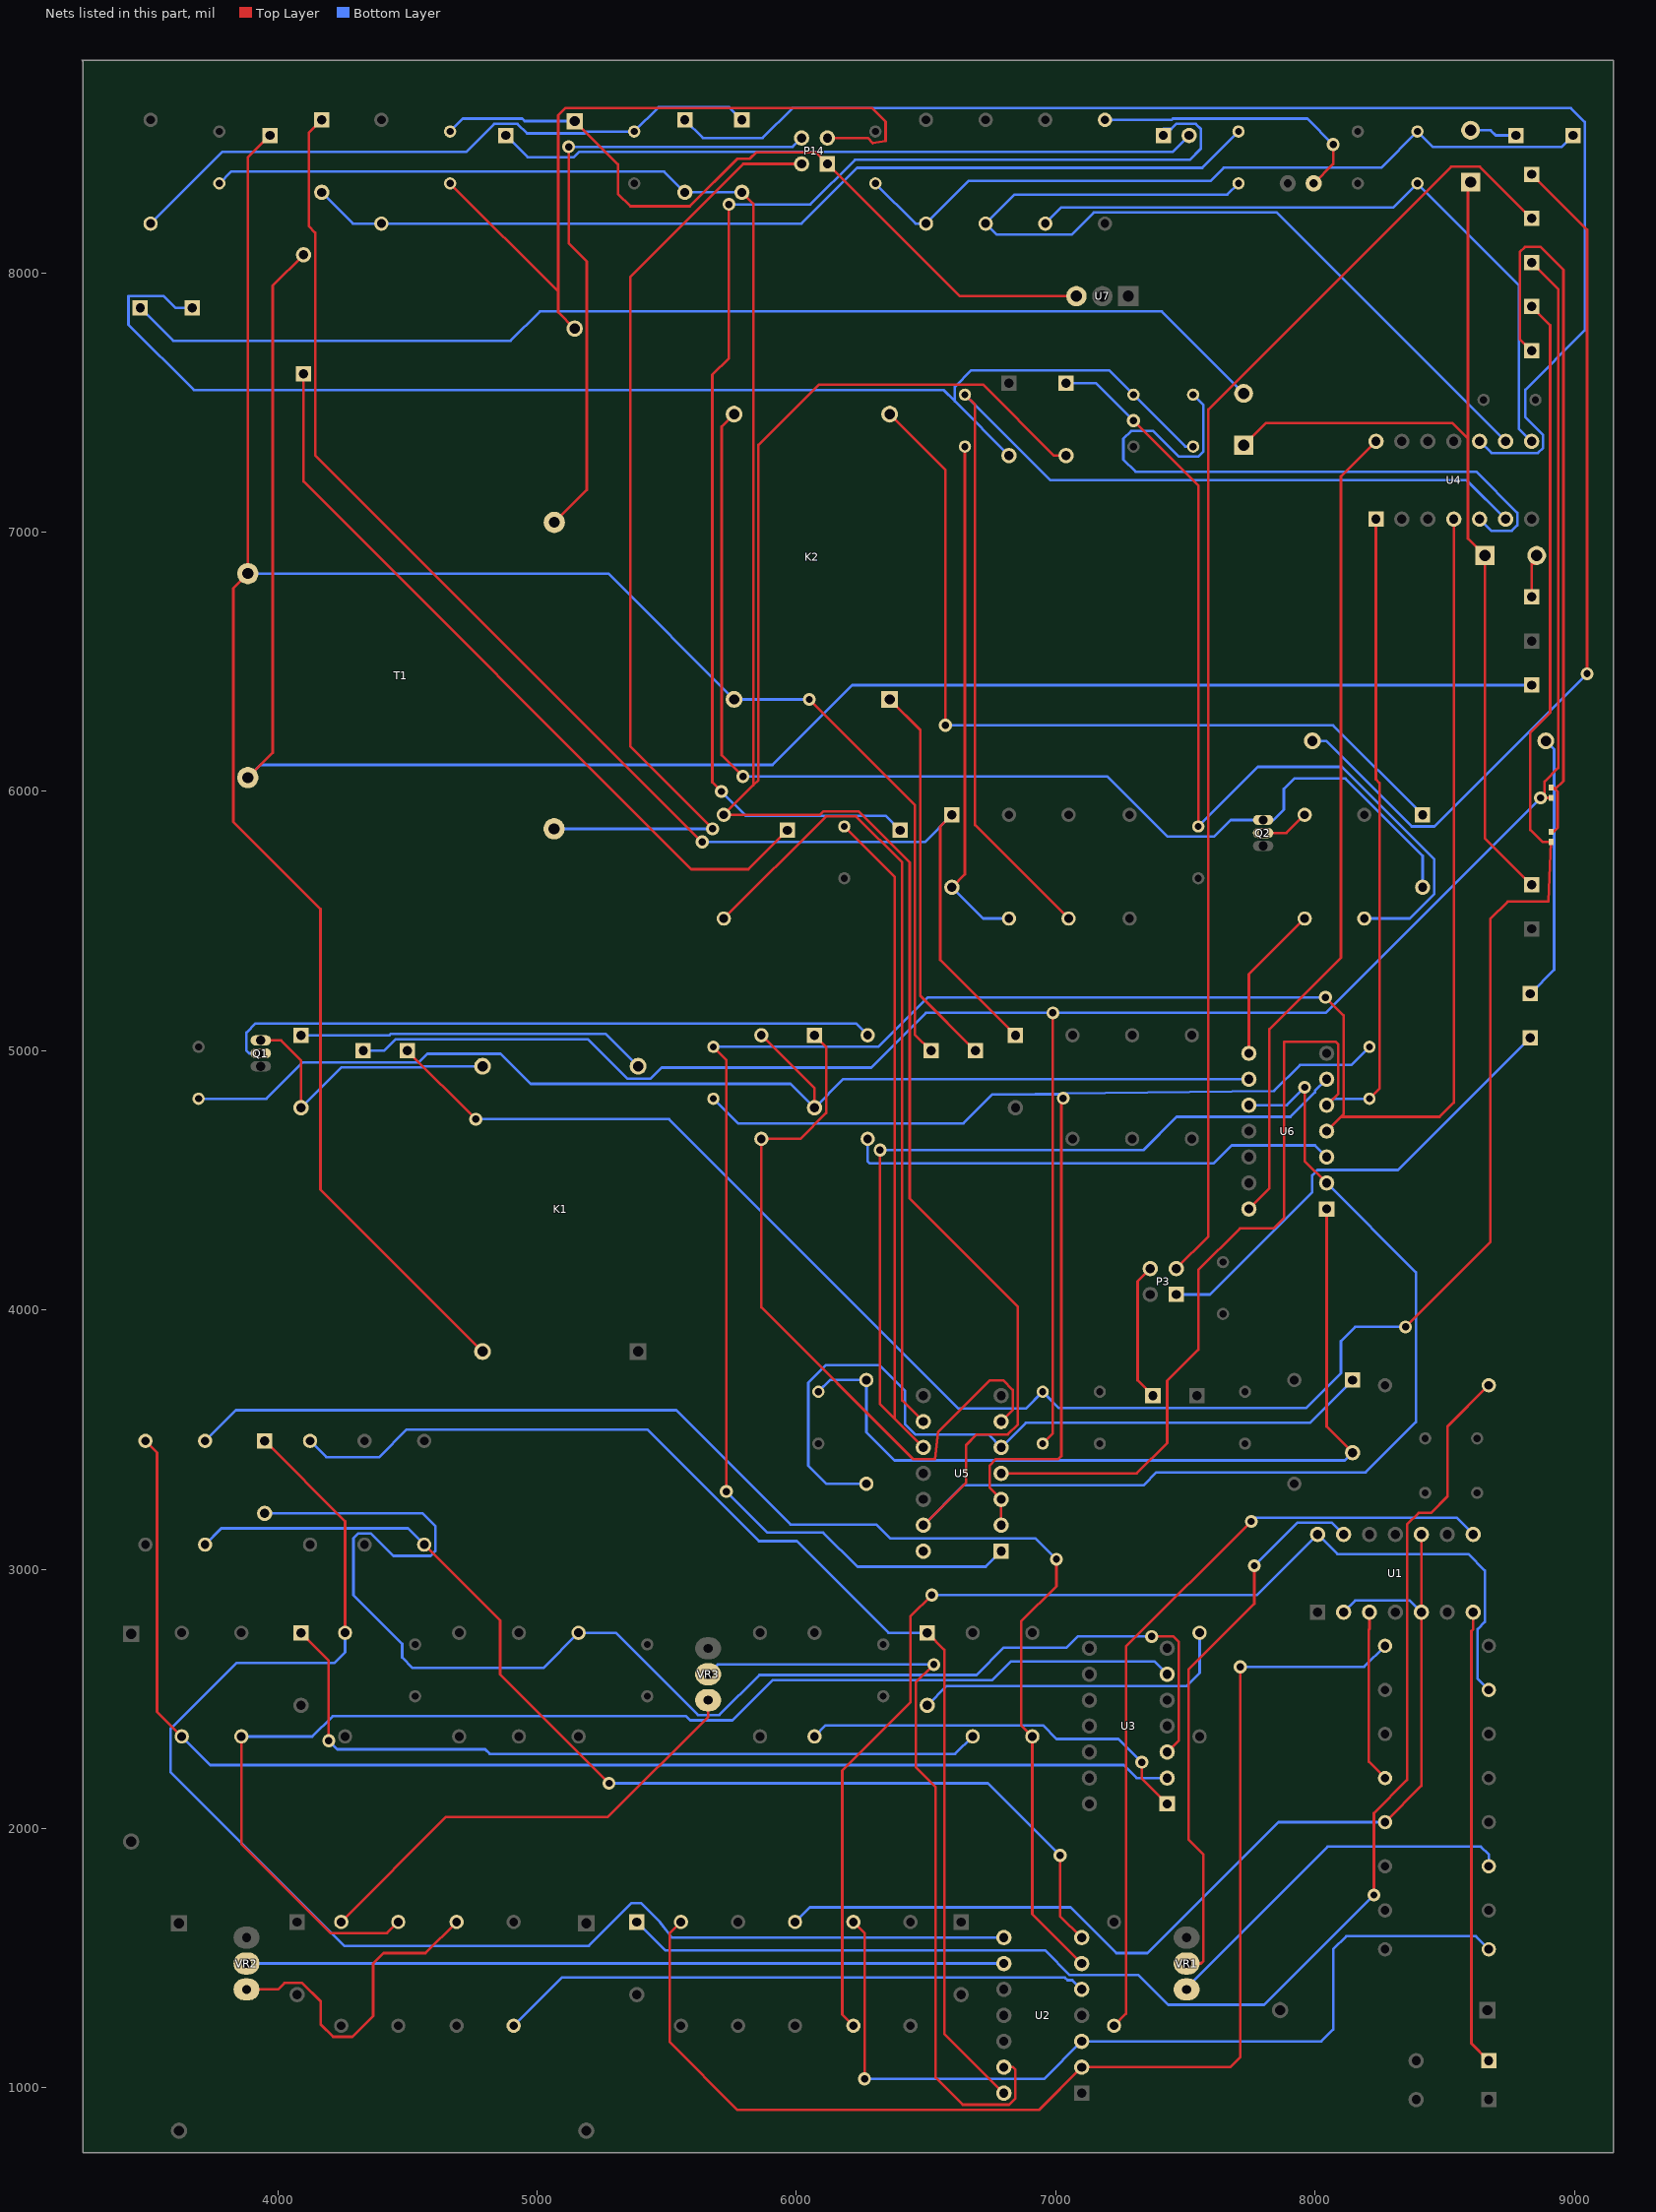
[diagram p0: the nets of this part, all layers, seen from the top]
# Altium PCB MISC82089.PcbDoc (part 2 of 2)
Units mil, origin at the board's own origin, x right, y up, seen from the top; angles counter-clockwise.
Board outline 5905 x 8070 mil, 2 copper layers (Top Layer, Bottom Layer); 156 components, 100 nets, 374 pads, 37 vias.

## Via types
v1: diameter 50, hole 28, Top Layer to Bottom Layer, 37 vias

## Nets (pads, with @x,y where several pads share a name; then routed paths per layer and width w, separated by ;. In a path a pad name is that pad's centre, name@x,y a point inside that pad or via, vN(x,y) a via of type N, cw(c..) or ccw(c..) an arc to the next point about the centre after c; other vN are vias at no path point) (continued)
NetC14_1: C14.1 L2.2 P6.1 P9.1 | length 8916.4
  Top Layer w10: C14.1@6950,3485 6989,3524 v1(6989,5146) ; P6.1@8835,8040 8938,7937 8938,6091 8885,6038 v1@8885,5975.31 ; v1(8870,5975.31) v1@8885,5975.31 ; L2.2@8910,5975.31 v1@8885,5975.31
  Bottom Layer w10: P9.1@4330,5000 4410.47,5000 4455,5044.53 5196.47,5044.53 5348.48,4892.52 5438,4892.52 5480.48,4935 6289,4935 6500,5146 v1(6989,5146) 8040.69,5146 v1(8870,5975.31)
NetC14_2: C14.2 L3.2 P7.1 P10.1 | length 9045.1
  Top Layer w10: P10.1@4500,5000 v1(4764,4736) ; v1(8349,3935) 8676,4262 8676,5508 8743,5575 8900,5575 L3.2@8910,5805.31 8876.69,5805.31 8830,5852 8830,6227 8907,6304 8907,7798 P7.1@8835,7870
  Bottom Layer w10: v1(4764,4736) 5509,4736 6625,3620 6885,3620 C14.2@6950,3685 7013,3622 7965,3622 8100,3757 8100,3880 8155,3935 v1(8349,3935)
NetC15_1: C15.1 U4.1 U5.4 U6.5 | length 5397.6
  Top Layer w10: U5.4@6790,3370 7313,3370 7430,3487 7430,3727 7550,3847 7550,4154 7710.62,4314.62 7840,4314.62 7881,4355.62 7881,5034 7882,5035 8080,5035 8090,5025 8090,4835 U6.5@8045,4790 ; C15.1@8210,4815 8249,4854 8249,6033 8235,6047 U4.1@8235,7050
  Bottom Layer w10: U6.5@8045,4790 8070,4815 C15.1@8210,4815
NetC15_2: C15.2 C17.1 U5.2 U5.3 | length 4833.3
  Top Layer w10: U5.2@6790,3170 U5.3@6790,3270 6745,3315 6745,3400 6770,3425 7010,3425 7022,3437 7022,4810 v1(7029,4817)
  Bottom Layer w10: C17.1@5680,4815 5775,4720 6644,4720 6756,4832 6812,4832 ; v1(7029,4817) 7014,4832 6812,4832 ; C15.2@8210,5015 8140,4945 7942,4945 7842,4845 7028.78,4834.74 6812,4832
NetC16_2: C16.2 D9.1 R37.2 U6.1 | length 3318.5
  Top Layer w10: U6.1@8045,4390 8045,3550.24 D9.1@8145,3450.24
  Bottom Layer w10: C16.2@6085,3685 6130,3730 R37.2@6270,3730 6270,3529 6379,3420 8114.76,3420 D9.1@8145,3450.24
NetC17_2: C17.2 U4.4 U5.1 U6.4 | length 8659.5
  Top Layer w10: C17.2@5680,5015 5730,4965 v1(5730,3300) ; v1(8040,5206) 8110,5136 8110,4755 8100,4745 ; U6.4@8045,4690 8100,4745 ; U4.4@8535,7050 8535,4800 8480,4745 8100,4745
  Bottom Layer w10: C17.2@5680,5015 6316,5015 6507,5206 v1(8040,5206) ; v1(5730,3300) 5888,3142 6104,3142 6236,3010 6730,3010 U5.1@6790,3070
NetC18_1: C18.1 D11.1 R41.2 U6.9 | length 4617.9
  Top Layer w10: R41.2@5865,5060 6070,4855 D11.1@6070,4780.24
  Bottom Layer w10: C18.1@3695,4815 3957,4815 4097.47,4955.47 4545,4955.47 4577.53,4988 4860,4988 4975.48,4872.52 5977.72,4872.52 D11.1@6070,4780.24 6179.76,4890 U6.9@7745,4890
NetC19_1: C19.1 C20.2 D13.1 J10.1 | length 5100.8
  Bottom Layer w10: J10.1@3670,7865 3606,7865 3561,7910 3425,7910 3425,7800 3677,7548 6567.24,7548 6611,7504.24 ; D13.1@6820,7295.24 6611,7504.24 ; C19.1@7530,7330 7500,7330 C20.2@7300,7530 7206,7624 6675,7624 6611,7560 6611,7504.24
NetC19_2: C19.2 U4.5 | length 2509.5
  Bottom Layer w10: C19.2@7530,7530 7569,7491 7569,7310 7550,7291 7475,7291 7376,7390 7291,7390 7261,7360 7261,7280 7308,7233 8621.53,7233 8780,7074.53 8780,7027 8758.47,7005.47 8679.53,7005.47 U4.5@8635,7050
NetC21_1: C21.1 D16.1 R47.1 | length 1990.3
  Top Layer w10: D16.1@6600,5630.24 6650,5680.24 C21.1@6650,7330
  Bottom Layer w10: D16.1@6600,5630.24 6720.24,5510 R47.1@6820,5510
NetC21_2: C21.2 R45.1 U4.6 | length 4469.5
  Top Layer w10: C21.2@6650,7530 6689,7491 6689,5871 R45.1@7050,5510
  Bottom Layer w10: C21.2@6650,7530 6980,7200 8585,7200 U4.6@8735,7050
NetC22_2: C22.2 D14.2 R43.1 | length 3584
  Top Layer w10: v1(7300,7430) 7550,7180 C22.2@7550,5865
  Bottom Layer w10: D14.2@7040,7574.76 7155.24,7574.76 v1(7300,7430) ; C22.2@7550,5865 7780,6095 8103,6095 8460,5738 8460,5605 8365,5510 R43.1@8190,5510
NetC23_2: C23.2 U5.10 U6.6 | length 5418.4
  Top Layer w10: C23.2@6185,5865 6379,5671 6379,3581 ; v1(6323,4617) 6323,3637 6379,3581 ; U5.10@6490,3470 6379,3581
  Bottom Layer w10: v1(6323,4617) 7338,4617 7466,4745 7904.78,4745 8000,4840.22 8000,4845 U6.6@8045,4890
NetC24_1: C24.1 R50.1 U4.8 | length 2676.5
  Bottom Layer w10: R50.1@6960,8190 7022.56,8252.56 8302.56,8252.56 C24.1@8395,8345 8786,7954 8786,7399 U4.8@8835,7350
NetC24_2: C24.2 C27.1 J12.1 R52.1 | length 2944.7
  Bottom Layer w10: C27.1@6305,8345 6460,8190 R52.1@6500,8190 6664,8354 7596.76,8354 7647.89,8405.13 8255.13,8405.13 C24.2@8395,8545 8455,8485 8950,8485 J12.1@8995,8530
NetC26_1: C26.1 R49.1 U4.9 | length 3462.7
  Bottom Layer w10: C26.1@7705,8345 7662,8302 6842,8302 R49.1@6730,8190 6772.56,8147.44 7061.88,8147.44 7147,8232.56 7852.44,8232.56 U4.9@8735,7350
NetC26_2: C26.2 D20.1 R53.1 | length 3731.8
  Bottom Layer w10: D20.1@4170,8310.24 4290.24,8190 R53.1@4400,8190 6020,8190 6235,8405 7565,8405 C26.2@7705,8545
NetC28_2: C28.2 D18.2 R54.1 | length 2516.6
  Bottom Layer w10: R54.1@3510,8190 3786,8466 4726.47,8466 4835,8574.53 4925,8574.53 4961.53,8538 5184,8538 5191,8545 C28.2@5375,8545 5469,8639 5740.76,8639 D18.2@5790,8589.76
NetC29_1: C29.1 C30.2 P14.1 U7.3 | length 2957.6
  Top Layer w10: C29.1@5145,8585 5312,8418 5312,8305 5360,8257 5589,8257 5772,8440 5821,8440 5846,8465 6075,8465 P14.1@6120,8420 6630,7910 U7.3@7080,7910
  Bottom Layer w10: C30.2@4665,8545 4714.53,8594.53 4943,8594.53 4952.53,8585 C29.1@5145,8585
NetC29_2: C29.2 C30.1 P14.3 | length 3041.5
  Top Layer w10: C30.1@4665,8345 5082,7928 ; C29.2@5145,7785 5082,7848 5082,7928 ; P14.3@6120,8520 6275,8520 6295,8500 6344,8509 6344,8583 6291,8636 5110,8636 5082,8608 5082,7928
NetC31_1: C31.1 D14.1 D18.1 D19.1 R48.2 U5.13 U6.2 U6.10 | length 14779.3
  Top Layer w10: D18.1@5790,8310.24 5834.15,8266.08 5834.15,6024.15 ; U5.13@6490,3170 6655,3335 6655,3480 6695,3520 6815,3520 6854.53,3559.53 6854.53,4012.47 6437,4430 6437,5726 6239.38,5923.62 6104.62,5923.62 6091,5910 R48.2@5720,5910 5834.15,6024.15 ; D14.1@7040,7295.24 6993.76,7295.24 6720,7569 6087,7569 5854,7336 5854,6044 5834.15,6024.15 ; v1(7960,4859) 7960,4575 U6.2@8045,4490
  Bottom Layer w10: C31.1@3775,8345 3820,8390 5490.24,8390 D19.1@5570,8310.24 D18.1@5790,8310.24 ; U5.13@6490,3170 6645,3325 7340,3325 7389,3374 8195,3374 8389,3568 8389,4146 U6.2@8045,4490 ; U6.10@7745,4790 7891,4790 v1(7960,4859)
NetD1_2: D1.2 U1.7 | length 1760.6
  Top Layer w10: U1.7@8610,2835 8610,2769 8603,2762 8603,1171.76 D1.2@8669.76,1105
NetD4_2: D4.2 R9.2 | length 5326.3
  Top Layer w10: v1(8227,1744) 8227,2060 8355,2188 8355,3173 8400,3218 8447,3218 8511,3282 8511,3551 R9.2@8670,3710
  Bottom Layer w10: D4.2@5385,1639.76 5494.76,1530 6960.47,1530 7055,1435.47 7319.53,1435.47 7434,1321 7804,1321 v1(8227,1744)
NetD6_1: D6.1 R30.2 U3.3 | length 5456.2
  Top Layer w10: v1(7370,2741) 7454,2741 7475,2720 7475,2340.5 U3.3@7430,2295.5
  Bottom Layer w10: D6.1@3950,3215.73 4559.27,3215.73 4608,3167 4608,3070 4590,3052 4446.06,3052 4360,3138.06 4310,3138.06 4292,3120.06 4292,2901 4480,2713 4480,2660 4520,2620 5024.5,2620 R30.2@5160,2755.5 5303.5,2755.5 5621,2438 5703,2438 5857.75,2592.75 6695.19,2592.75 6800.44,2698 7042,2698 7085,2741 v1(7370,2741)
NetD6_2: D6.2 R33.2 U2.8 | length 5524.2
  Top Layer w10: D6.2@3950,3495.26 4260,3185.26 R33.2@4260,2755.5
  Bottom Layer w10: R33.2@4260,2755.5 4260,2680 4219.06,2639.06 3841,2639.06 3587.44,2385.5 3587.44,2217.56 4257,1548 5200,1548 5365,1713 5401,1713 5474,1640 5520,1580 U2.8@6800,1580
NetD7_1: D7.1 R24.2 | length 1257
  Bottom Layer w10: D7.1@6505,2475.73 6579.27,2550 7505,2550 7555,2600 R24.2@7555,2755.5
NetD7_2: D7.2 R21.2 U2.14 | length 4671.9
  Top Layer w10: D7.2@6505,2755.26 6570.47,2689.79 6570.47,1209.53 U2.14@6800,980
  Bottom Layer w10: R21.2@4125,3495.5 4187.56,3432.94 4392.03,3432.94 4498.09,3539 5426,3539 5856,3109 6002,3109 6355.74,2755.26 D7.2@6505,2755.26
NetD8_2: D8.2 R27.1 | length 2992.7
  Top Layer w10: D8.2@4090,2755.26 4197,2648.26 v1(4197,2339)
  Bottom Layer w10: v1(4197,2339) 4230,2306 4800,2306 4818,2288 6612.5,2288 R27.1@6680,2355.5
NetD9_2: D9.2 R37.1 U5.5 | length 3015
  Bottom Layer w10: R37.1@6270,3330 6116,3330 6046,3400 6046,3720 6114,3788 6320,3788 6419,3689 6419,3560 6459,3520 6740,3520 U5.5@6790,3470 6885,3565 7980.24,3565 D9.2@8145,3729.76
NetD10_2: D10.2 D16.2 D20.2 | length 5429
  Top Layer w10: D20.2@4170,8589.76 4120,8539.76 4120,8180 4145,8155 4145,7297 v1(5637,5805) ; D16.2@6600,5909.76 6555,5864.76 6555,5349.76 D10.2@6845,5059.76
  Bottom Layer w10: v1(5637,5805) 6495.24,5805 D16.2@6600,5909.76
NetD11_2: D11.2 R41.1 U5.6 | length 2802.9
  Top Layer w10: D11.2@6070,5059.76 6115,5014.76 6115,4760 6015,4660 R41.1@5865,4660 5865,4010 6449.53,3425.47 6535,3425.47 6546,3528 6747,3729 6798,3729 6834.53,3692.47 6834.53,3614.53 U5.6@6790,3570
NetD12_1: D12.1 K1.4 Q1.3 | length 1135.8
  Top Layer w10: Q1.3@3935,5040 4013,5040 4090,4963 D12.1@4090,4780.24
  Bottom Layer w10: D12.1@4090,4780.24 4245.24,4935.47 4558,4935.47 4562.53,4940 K1.4@4790,4940
NetD12_2: D12.2 K1.3 | length 1353.6
  Bottom Layer w10: D12.2@4090,5059.76 4430.71,5059.76 4435.47,5064.53 5265.47,5064.53 K1.3@5390,4940
NetD15_1: D15.1 K2.4 Q2.3 | length 4552.8
  Top Layer w10: K2.4@5760,7455 5712,7407 5712,6140 v1(5794,6058)
  Bottom Layer w10: v1(5794,6058) 7199,6058 7431,5826 7611,5826 7675,5890 Q2.3@7800,5890 7840,5890 7880,5930 7880,6010 7920,6050 8117,6050 8415,5752 D15.1@8415,5630.24
NetD15_2: D15.2 K2.3 | length 3272.1
  Top Layer w10: K2.3@6360,7455 6575,7240 v1(6575,6255)
  Bottom Layer w10: v1(6575,6255) 8069.76,6255 D15.2@8415,5909.76
NetD17_2: D17.2 R51.2 | length 1104.2
  Top Layer w10: D17.2@7995,8345 8070,8420 v1(8070,8495)
  Bottom Layer w10: R51.2@7190,8590 7447.47,8590 7452,8594.53 7970.47,8594.53 v1(8070,8495)
NetD19_2: D19.2 U4.10 | length 5220.5
  Bottom Layer w10: D19.2@5570,8589.76 5639.76,8520 5870,8520 5985,8635 8987,8635 9040,8582 9040,7778 8811,7549 8811,7443 8879.53,7374.47 8879.53,7324.53 8860,7305 8680,7305 U4.10@8635,7350
NetF1_1: F1.1 J11.1 | length 2962.1
  Top Layer w10: F1.1@4100,7610.67 4100,7195 5595,5700 5815,5700 J11.1@5965,5850
NetF1_2: F1.2 J4.1 T1.4 | length 7202.8
  Top Layer w10: T1.4@3885,6053.33 3981,6149.33 3981,7950.33 F1.2@4100,8069.33
  Bottom Layer w10: T1.4@3885,6053.33 3934.06,6102.39 5908.09,6102.39 6215.7,6410 J4.1@8835,6410
NetJ1_1: J1.1 P3.1 | length 1813.7
  Bottom Layer w10: P3.1@7465,4060 7595,4060 7989,4454 7989,4520 8009,4540 8320,4540 J1.1@8830,5050
NetJ5_1: J5.1 P3.3 | length 5080.5
  Top Layer w10: P3.3@7465,4160 7589,4284 7589,7473 8525,8409 8636,8409 J5.1@8835,8210
NetJ6_1: J6.1 P3.4 | length 534.7
  Top Layer w10: P3.4@7365,4160 7316,4111 7316,3729 J6.1@7375,3670
NetJ8_1: J8.1 J13.1 K1.2 K2.2 T1.3 | length 9062
  Top Layer w10: J13.1@3970,8530 3885,8445 T1.3@3885,6840 3829,6784 3829,5883 4165,5547 4165,4465 K1.2@4790,3840 ; v1(6050,6355) 6457,5948 6457,5063 J8.1@6520,5000
  Bottom Layer w10: T1.3@3885,6840 5275,6840 K2.2@5760,6355 v1(6050,6355)
NetJ9_1: J9.1 K2.1 | length 1491.7
  Top Layer w10: K2.1@6360,6355 6478,6237 6478,5212 J9.1@6690,5000
NetL1_1: L1.1 P8.1 | length 3454.3
  Top Layer w10: P8.1@8835,8380 9049,8166 v1(9049,6454)
  Bottom Layer w10: L1.1@7990,6195 8043,6195 8373,5865 8460,5865 v1(9049,6454)
NetL1_2: L1.2 P1.1 | length 1026.4
  Bottom Layer w10: P1.1@8830,5220 8922,5312 8922,6163 L1.2@8890,6195
NetL2_1: L2.1 L3.1 P5.1 | length 2848.2
  Top Layer w10: P5.1@8835,7700 8790,7745 8790,8080 8810,8100 8870,8100 8958,8012 8958,6040 8926.5,6008.5 ; L3.1@8910,5844.69 8920,5844.69 8935,5859.69 8935,6000 8926.5,6008.5 ; 8926.5,6008.5 8920.31,6014.69 L2.1@8910,6014.69 8926.5,6008.5
NetLS1_1: LS1.1 P12.1 | length 5227.1
  Top Layer w10: v1(5711,6000) 5676,6035 5676,7607 5740,7671 v1(5740,8264)
  Bottom Layer w10: v1(5711,6000) 5805,5906 6344,5906 P12.1@6400,5850 ; v1(5740,8264) 6054,8264 6226,8436 7517,8436 7560,8479 7560,8554.53 7540,8574.53 7465,8574.53 7445.47,8555 7415,8555 LS1.1@7415,8530
NetLS1_2: LS1.2 P15.1 | length 2704.6
  Bottom Layer w10: P15.1@4880,8530 4964.01,8445.99 5142.23,8445.99 5162.24,8466 7451,8466 LS1.2@7515,8530
NetP2_1: P2.1 S1.1 S2.1 S3.1 | length 3747.4
  Top Layer w10: S2.1@7725,7335 7811,7421 8529,7421 8590,7360 ; S3.1@8600,8350 8600,8348 8590,8348 8590,7360 ; P2.1@8835,5640 8655,5820 S1.1@8655,6910 8590,6975 8590,7360
NetP4_1: P4.1 S1.2 | length 180
  Top Layer w10: P4.1@8835,6750 8835,6878.58 8855,6878.58 S1.2@8855,6910
NetP11_1: P11.1 S2.2 | length 4485.3
  Bottom Layer w10: P11.1@3470,7865 3597,7738 4898,7738 5011,7851 7409,7851 S2.2@7725,7535
NetP13_1: P13.1 S3.2 | length 183.3
  Bottom Layer w10: S3.2@8600,8550 8677,8550 8697,8530 P13.1@8775,8530
NetP14_2: P14.2 T1.1 | length 3711.7
  Top Layer w10: v1(5677,5856) 5360,6173 5360,7985 5795,8420 P14.2@6020,8420
  Bottom Layer w10: T1.1@5065.83,5855.83 5676.83,5855.83 v1(5677,5856)
NetP14_4: P14.4 T1.2 | length 2441.5
  Top Layer w10: T1.2@5066.67,7037.5 5192,7162.83 5192,8044 5122,8114 v1(5122,8486)
  Bottom Layer w10: v1(5122,8486) 5986,8486 P14.4@6020,8520
NetQ1_2: Q1.2 R42.2 | length 2557.3
  Bottom Layer w10: Q1.2@3935,4990 3890,4990 3880,5000 3880,5070 3915,5105 6230,5105 R42.2@6275,5060
NetQ2_2: Q2.2 R44.2 | length 189
  Top Layer w10: Q2.2@7800,5840 7890,5840 R44.2@7960,5910
NetR2_2: R2.2 R12.2 U2.3 | length 3459.9
  Top Layer w10: R12.2@6220,1640 6263,1597 v1(6263,1035)
  Bottom Layer w10: v1(6263,1035) 6955,1035 U2.3@7100,1180 8025,1180 8070,1225 8070,1535 8120,1585 8620,1585 R2.2@8670,1535
NetR4_1: R4.1 U1.3 | length 667
  Top Layer w10: U1.3@8210,2835 8210,2770.12 8207.44,2767.56 8207.44,2257.56 R4.1@8270,2195
NetR5_1: R5.1 R13.2 U1.2 U1.5 U1.10 | length 4086.2
  Top Layer w10: R5.1@8270,2025 8410,2165 U1.5@8410,2835 U1.10@8410,3135
  Bottom Layer w10: R13.2@5995,1640 6051.84,1696.84 7057.16,1696.84 7234,1520 7354,1520 7859,2025 R5.1@8270,2025 ; U1.2@8110,2835 8155,2880 8365,2880 U1.5@8410,2835
NetR6_2: R6.2 VR1.1 | length 1455.8
  Bottom Layer w10: VR1.1@7505,1380 7505,1387 8049,1931 8640,1931 8670,1901 R6.2@8670,1855
NetR7_2: R7.2 R12.1 U1.14 | length 4599
  Top Layer w10: R12.1@6220,1240 6177,1283 6177,2224 6440.47,2487.47 6440.47,2819.47 v1(6522,2901)
  Bottom Layer w10: v1(6522,2901) 7776,2901 U1.14@8010,3135 8086,3059 8591,3059 8655,2995 8655,2797 8627,2769 8627,2578 R7.2@8670,2535
NetR8_1: R8.1 R15.2 U2.2 | length 4969.4
  Top Layer w10: R15.2@5555,1640 5512,1597 5512,1177 5773.53,915.47 6935.47,915.47 U2.2@7100,1080 7672,1080 7712,1120 v1(7712,2624)
  Bottom Layer w10: v1(7712,2624) 8189,2624 R8.1@8270,2705
NetR10_1: R10.1 U1.8 | length 3052.9
  Top Layer w10: R10.1@7225,1240 7271,1286 7271,2702 v1(7754,3185)
  Bottom Layer w10: v1(7754,3185) 7768.53,3199.53 8545.47,3199.53 U1.8@8610,3135
NetR16_1: R16.1 U2.5 | length 2286.1
  Bottom Layer w10: R16.1@4910,1240 5096,1426 7035.47,1426 7046,1415.47 7064.53,1415.47 U2.5@7100,1380
NetR17_2: R17.2 VR2.1 | length 1260.2
  Top Layer w10: VR2.1@3880,1380 4001,1380 4026,1405 4094.53,1405 4166,1333.53 4166,1245 4213.56,1197.44 4288,1197.44 4368,1277.44 4368,1480 4408,1520 4570,1520 R17.2@4690,1640
NetR18_2: R18.2 VR3.1 | length 1806.6
  Top Layer w10: R18.2@4245,1640 4650,2045 5273,2045 5660,2432 VR3.1@5660,2495.5
NetR19_2: R19.2 R35.1 U3.6 | length 4903.6
  Top Layer w10: R35.1@3860,2355.5 3860,1940.76 4203.76,1597 4422,1597 R19.2@4465,1640
  Bottom Layer w10: R35.1@3860,2355.5 4133.52,2355.5 4212.02,2434 5575,2434 5591,2418 5754,2418 5908.75,2572.75 6755.72,2572.75 6827.97,2645 7380.5,2645 U3.6@7430,2595.5
NetR20_1: R20.1 R23.1 U2.7 | length 4318.2
  Top Layer w10: R20.1@4565,3095.5 4858,2802.5 4858,2595 v1(5278,2175) ; v1(7017,1897) 7017,1663 U2.7@7100,1580
  Bottom Layer w10: R23.1@3720,3095.5 3782.56,3158.06 4502.44,3158.06 R20.1@4565,3095.5 ; v1(5278,2175) 6739,2175 v1(7017,1897)
NetR23_2: R23.2 R26.1 U2.6 | length 5282.1
  Top Layer w10: v1(7003,3039) 7003,2935 6867,2799 6867,2398.5 R26.1@6910,2355.5 6910,1670 U2.6@7100,1480
  Bottom Layer w10: R23.2@3720,3495.5 3838.5,3614 5537,3614 5978,3173 6309,3173 6362,3120 6922,3120 v1(7003,3039)
NetR25_2: R25.2 R34.1 U3.2 | length 5064.3
  Top Layer w10: R25.2@3490,3495.5 3535,3450.5 3535,2450.5 R34.1@3630,2355.5
  Bottom Layer w10: R34.1@3630,2355.5 3740.5,2245 7262.44,2245 7311.95,2195.5 U3.2@7430,2195.5
NetR28_1: R28.1 U3.1 | length 1539.6
  Top Layer w10: v1(7332,2256) 7332,2193.5 U3.1@7430,2095.5
  Bottom Layer w10: R28.1@6070,2355.5 6112.56,2398.06 6950.94,2398.06 7003,2346 7242,2346 v1(7332,2256)
NetR42_1: R42.1 U6.3 | length 1907.7
  Bottom Layer w10: R42.1@6275,4660 6275,4573.1 6282.86,4565.24 7609.24,4565.24 7679,4635 8000,4635 U6.3@8045,4590
NetR44_1: R44.1 U6.8 | length 609.1
  Top Layer w10: U6.8@7745,4990 7745,5295 R44.1@7960,5510
NetR48_1: R48.1 U5.9 | length 3115
  Top Layer w10: R48.1@5720,5510 6113.62,5903.62 6231.09,5903.62 6408,5726.71 6408,3652 U5.9@6490,3570
NetU1_13: U1.13 VR1.2 | length 2153.4
  Top Layer w10: VR1.2@7505,1480 7560,1480 7570,1490 7570,1900 7512,1958 7512,2613 7766,2867 v1(7766,3014)
  Bottom Layer w10: v1(7766,3014) 7931.53,3179.53 8065.47,3179.53 U1.13@8110,3135
NetU2_9: U2.9 VR2.2 | length 2920
  Bottom Layer w10: VR2.2@3880,1480 U2.9@6800,1480
NetU2_13: U2.13 VR3.2 | length 3060.5
  Top Layer w10: v1(6530,2633) 6460.47,2563.47 6460.47,2237 6537,2160.47 6537,1040 6641.53,935.47 6820.47,935.47 6845,960 6845,1070 6835,1080 U2.13@6800,1080
  Bottom Layer w10: VR3.2@5660,2595.5 5660,2597 5696,2633 v1(6530,2633)
VCC: U4.14 U6.14 | length 3163
  Top Layer w10: U6.14@7745,4390 7824,4469 7824,5083 8100,5359 8100,7215 U4.14@8235,7350
VDD: U5.14
pads on no net: C7.1 D2.2 D5.2 K1.1 R3.1 R16.2 R38.2 R46.1 R47.2 R53.2 U1.4 U1.6 U1.11 U3.7 U3.8 U3.9 U3.10 U3.12 U3.13 U3.14 U4.11 U4.12 U4.13 U5.8 U6.11 U6.12 U6.13 VR1.3 VR2.3 VR3.3

## Polygon pours and split planes (outlines as drawn)
GND on Top Layer "D" (solid, remove dead copper, pour order 0): 2685,9475 10305,9475 10320,9490 9635,8805 9635,425 3065,425 2830,190
GND on Bottom Layer "D" (solid, remove dead copper, pour order 2): 2085,9505 2230,9650 10455,9650 10455,805 9855,205 9740,320 2640,320

## Keep-outs
Keep-Out Layer:
  lines w10: 3245,8820 cw(c3232.93,8807.93) 3250,8807.93 3250,8750 3250,750 8860,750 9150,750 9150,8820 3245,8820